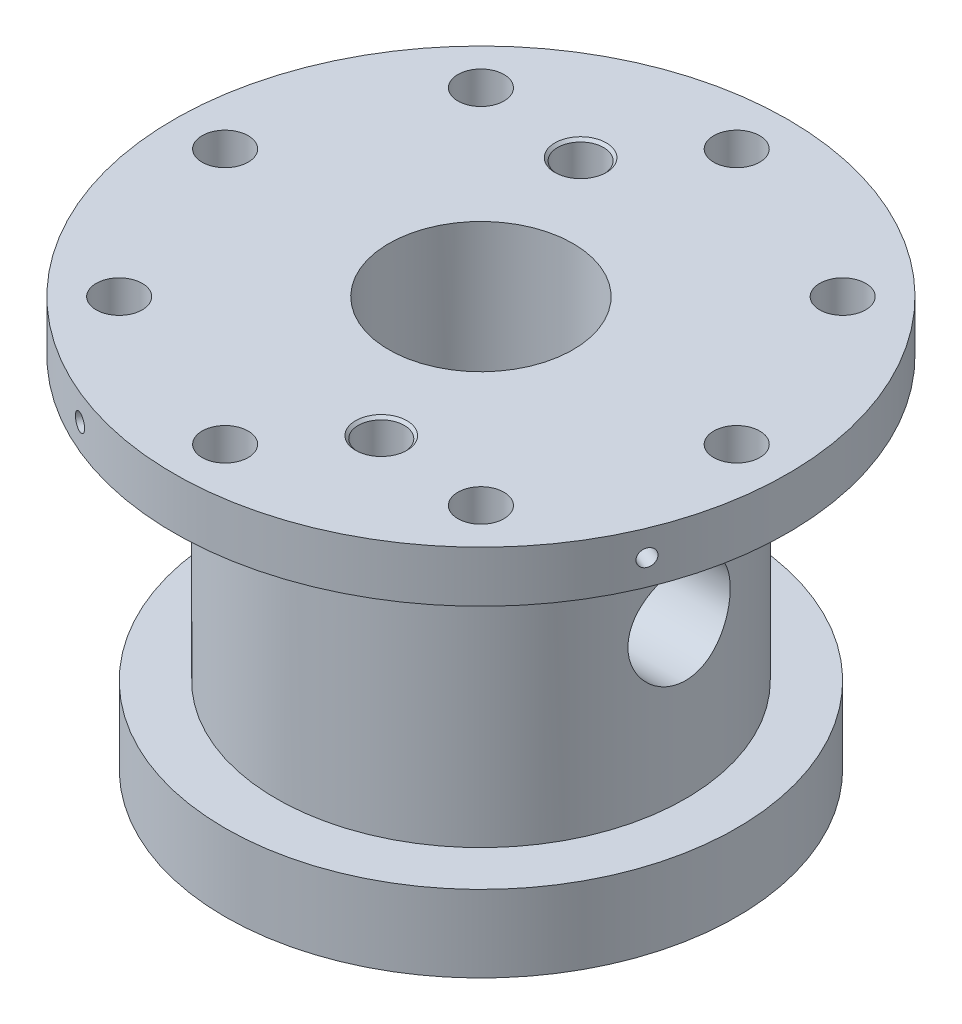
SolidWorks part; units mm, degrees
ref_plane "前视基准面" through (0, 0, 0) normal (0, 0, 1) x (1, 0, 0)
ref_plane "上视基准面" through (0, 0, 0) normal (0, 1, 0) x (1, 0, 0)
ref_plane "右视基准面" through (0, 0, 0) normal (1, 0, 0) x (0, 0, -1)
sketch "草图1" plane through (0, 0, 0) normal (0, 0, 1) x (1, 0, 0)
  line L0 (0, 0) -> (0, 60) construction
  line L1 (18, 60) -> (60, 60)
  line L2 (60, 60) -> (60, 50)
  line L3 (60, 50) -> (40, 50)
  line L4 (40, 50) -> (40, 0)
  line L5 (40, 0) -> (18, 0)
  line L6 (18, 0) -> (18, 60)
  dimension "D1" = 18
  dimension "D2" = 40
  dimension "D3" = 60
  dimension "D4" = 60
  dimension "D5" = 50
revolve "旋转1" add sketch "草图1" angle 360 about L0
sketch "草图2" plane through (0, 60, 0) normal (0, 1, 0) x (1, 0, 0)
  line L0 (0, 0) -> (0, 50) construction
  circle A0 centre (0, 50) radius 4.5
  dimension "D2" = 9
  dimension "D1" = 50
extrude "切除-拉伸1" cut sketch "草图2" against normal blind 10
pattern_circular "阵列(圆周)1" count 8 over 360 about axis through (0, 0, 0) along (0, 1, 0) of "切除-拉伸1"
sketch "草图3" plane through (0, 0, 0) normal (0, -1, 0) x (1, 0, 0)
  circle A1 centre (0, 0) radius 40
  circle A2 centre (0, 0) radius 40
  dimension "D1" = 0
extrude "凸台-拉伸1" add sketch "草图3" along normal blind 10
sketch "草图7" plane through (0, 0, 0) normal (0, 1, 0) x (1, 0, 0)
  circle A1 centre (0, 0) radius 18
  circle A2 centre (0, 0) radius 18
  dimension "D1" = 0
extrude "凸台-拉伸2" add sketch "草图7" along normal blind 10
sketch "草图5" plane through (0, -10, 0) normal (0, -1, 0) x (1, 0, 0)
  line L0 (0, 22) -> (0, 0) construction
  line L1 (2.5, 7) -> (-2.5, 7)
  line L2 (2.5, 7) -> (2.5, 37)
  line L3 (2.5, 37) -> (-2.5, 37)
  line L4 (-2.5, 7) -> (-2.5, 37)
  line L5 (2.5, 7) -> (-2.5, 37) construction
  line L6 (2.5, 37) -> (-2.5, 7) construction
  point P0 (0, 22)
  dimension "D1" = 30
  dimension "D2" = 5
  dimension "D3" = 22
extrude "切除-拉伸2" cut sketch "草图5" against normal blind 15
pattern_circular "阵列(圆周)3" count 3 over 360 about axis through (0, 0, 0) along (0, 1, 0) of "切除-拉伸2"
sketch "草图8" plane through (0, 60, 0) normal (0, 1, 0) x (1, 0, 0)
  line L0 (0, 0) -> (0, 39.8939) construction
  line L1 (0, 39.8939) -> (11.5032, 27.7711) construction
  line L2 (11.5032, 27.7711) -> (0, 0) construction
  dimension "D1" = 22.5
ref_plane "基准面1" through (0, 0, 0) normal (-0.9239, 0, -0.3827) x (-0.3827, 0, 0.9239)
sketch "草图9" plane through (0, 0, 0) normal (-0.9239, 0, -0.3827) x (-0.3827, 0, 0.9239)
  line L0 (-60, 60) -> (-60, 55)
  line L1 (-60, 60) -> (-60, 50) construction
  line L2 (-60, 55) -> (-60, 50)
hole_wizard "M4x0.7 螺纹孔1" positions "3D草图1" profile "草图10" tap size "M4x0.7" standard "BSI"
sketch3d "3D草图1"
  point P0 (22.961, 55, -55.4328)
sketch "草图10" plane through (22.961, 55, -55.4328) normal (0, 1, 0) x (-0.9239, 0, -0.3827)
  line L0 (0, 0) -> (0, 11.0914)
  line L1 (0, 11.0914) -> (1.65, 10.1)
  line L2 (1.65, 10.1) -> (1.65, 0)
  line L5 (1.65, 0) -> (0, 0)
  line L10 (0, 11.0914) -> (-1.65, 10.1) construction
  line L11 (0, -6.35) -> (0, 107.95) construction
  dimension "螺纹孔钻头直径" = 3.3
  dimension "螺纹孔钻头深度" = 10.1
  dimension "导头角度" = 118
cosmetic thread "孔螺蚊线1" parameters "D1"=8, "D2"=4
pattern_circular "阵列(圆周)4" count 4 over 360 about axis through (0, 0, 0) along (0, -1, 0) of "M4x0.7 螺纹孔1"
cosmetic thread "孔螺蚊线2" parameters "D1"=8, "D2"=4
cosmetic thread "孔螺蚊线3" parameters "D1"=8, "D2"=4
cosmetic thread "孔螺蚊线4" parameters "D1"=8, "D2"=4
sketch "草图11" plane through (0, -10, 0) normal (0, -1, 0) x (1, 0, 0)
  line L37 (-2.5, 37) -> (-2.5, 7)
  line L38 (2.5, 37) -> (-2.5, 37)
  line L39 (2.5, 7) -> (2.5, 37)
  line L40 (-2.5, 7) -> (2.5, 7)
  line L41 (-2.5, 37) -> (-2.5, 7)
  line L42 (2.5, 37) -> (-2.5, 37)
  line L43 (2.5, 7) -> (2.5, 37)
  line L44 (-2.5, 7) -> (2.5, 7)
  line L45 (33.2929, -16.3349) -> (7.3122, -1.3349)
  line L46 (30.7929, -20.6651) -> (33.2929, -16.3349)
  line L47 (4.8122, -5.6651) -> (30.7929, -20.6651)
  line L48 (7.3122, -1.3349) -> (4.8122, -5.6651)
  line L49 (33.2929, -16.3349) -> (7.3122, -1.3349)
  line L50 (30.7929, -20.6651) -> (33.2929, -16.3349)
  line L51 (4.8122, -5.6651) -> (30.7929, -20.6651)
  line L52 (7.3122, -1.3349) -> (4.8122, -5.6651)
  line L53 (-30.7929, -20.6651) -> (-4.8122, -5.6651)
  line L54 (-33.2929, -16.3349) -> (-30.7929, -20.6651)
  line L55 (-7.3122, -1.3349) -> (-33.2929, -16.3349)
  line L56 (-4.8122, -5.6651) -> (-7.3122, -1.3349)
  line L57 (-30.7929, -20.6651) -> (-4.8122, -5.6651)
  line L58 (-33.2929, -16.3349) -> (-30.7929, -20.6651)
  line L59 (-7.3122, -1.3349) -> (-33.2929, -16.3349)
  line L60 (-4.8122, -5.6651) -> (-7.3122, -1.3349)
  circle A0 centre (0, 0) radius 50
  circle A1 centre (0, 0) radius 40
  circle A2 centre (0, 0) radius 40
  dimension "D6" = 100
  dimension "D1" = 0
  dimension "D2" = 0
  dimension "D3" = 0
  dimension "D5" = 0
extrude "凸台-拉伸3" add sketch "草图11" along normal blind 10 and the other way blind 5
sketch "草图12" plane through (0, 60, 0) normal (0, 1, 0) x (1, 0, 0)
  line L0 (0, 0) -> (-13.7766, 33.2597) construction
  line L1 (0, 0) -> (-26.7406, 0) construction
  line L2 (-35.3553, 35.3553) -> (0, 50) construction
  line L3 (-17.6777, 42.6777) -> (-13.7766, 33.2597) construction
  line L4 (0, 0) -> (13.7766, -33.2597) construction
  dimension "D1" = 36
  dimension "D2" = 36
hole_wizard "M10x1.0 螺纹孔1" positions "3D草图2" profile "草图13" tap size "M10x1.0" standard "BSI"
sketch3d "3D草图2"
  point P5 (-13.7766, 60, -33.2597)
  point P9 (13.7766, 60, 33.2597)
sketch "草图13" plane through (-13.7766, 60, -33.2597) normal (1, 0, 0) x (0, 0, 1)
  line L0 (0, 0) -> (0, 25.7039)
  line L1 (0, 25.7039) -> (4.5, 23)
  line L2 (4.5, 23) -> (4.5, 0.525)
  line L3 (4.5, 0.525) -> (5.025, 0)
  line L5 (5.025, 0) -> (0, 0)
  line L6 (-4.5, 0.525) -> (-5.025, 0) construction
  line L10 (0, 25.7039) -> (-4.5, 23) construction
  line L11 (0, -6.35) -> (0, 107.95) construction
  dimension "螺纹孔钻头直径" = 9
  dimension "螺纹孔钻头深度" = 23
  dimension "近端锥形沉头孔直径" = 10.05
  dimension "近端锥形沉头孔角度" = 90
  dimension "导头角度" = 118
cosmetic thread "孔螺蚊线5" parameters "D1"=20, "D2"=10
cosmetic thread "孔螺蚊线6" parameters "D1"=20, "D2"=10
sketch "草图16" plane through (0, 0, 0) normal (1, 0, 0) x (0, 0, -1)
  line L0 (0, 25) -> (0, -5) construction
  line L1 (50, -5) -> (-50, -5) construction
  circle A0 centre (0, 25) radius 10
  dimension "D1" = 30
  dimension "D2" = 20
extrude "切除-拉伸3" cut sketch "草图16" against normal mid plane 130
